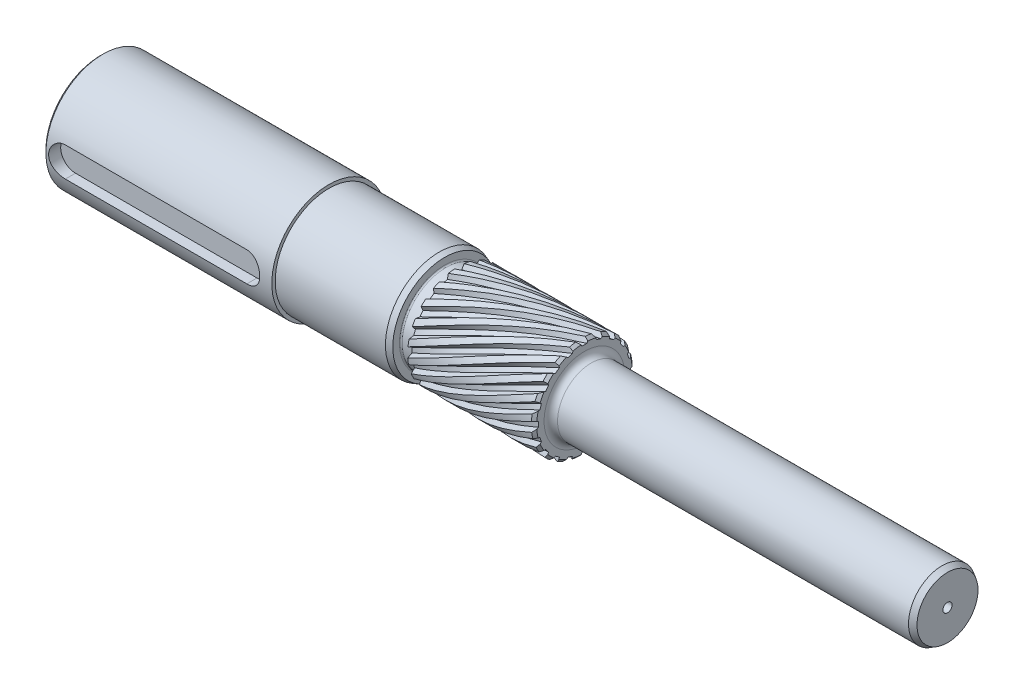
from build123d import *

# Parameters (mm, degrees)
SKETCH_1_R               = 42.5
EXTRUDE_1_DEPTH          = 360
SKETCH_17_OUTSIDE_W      = 162.908
SKETCH_17_OUTSIDE_H      = 162.908
SKETCH_17_OUTSIDE_R      = 40
CUT_EXTRUDE_6_DEPTH      = 190
SKETCH_4_OUTSIDE_W       = 162.908
SKETCH_4_OUTSIDE_H       = 162.908
SKETCH_4_OUTSIDE_R       = 32.5
CUT_EXTRUDE_2_DEPTH      = 10
SKETCH_19_OUTSIDE_W      = 162.908
SKETCH_19_OUTSIDE_H      = 162.908
SKETCH_19_OUTSIDE_R      = 37.5
CUT_EXTRUDE_7_DEPTH      = 94
SKETCH_14_OUTSIDE_W      = 162.908
SKETCH_14_OUTSIDE_H      = 162.908
SKETCH_14_OUTSIDE_R      = 42.5
CUT_EXTRUDE_4_DEPTH      = 360
CUT_EXTRUDE_5_DEPTH      = 9
CHAMFER_1_SIZE           = 2
FILLET_1_R               = 1
CHAMFER_2_SIZE           = 4
CHAMFER_2_SIZE2          = 1.455880937
EXTRUDE_START            = -360
SKETCH_20_R              = 25
EXTRUDE_2_DEPTH          = 270
CHAMFER_3_SIZE           = 4
CHAMFER_3_SIZE2          = 2.309401077
FILLET_2_R               = 5
HOLE_WIZARD_M8_1_D       = 6.8
HOLE_WIZARD_M8_1_DEPTH   = 19.75
HOLE_WIZARD_M8_1_TIP     = 2.042926105
CHAMFER_4_SIZE           = 2
SWEEP_1_PITCH            = 480
SWEEP_1_HEIGHT           = 94
SWEEP_1_RADIUS           = 36
SWEEP_1_START_ANGLE      = -90
PATTERN_CIRCULAR_2_COUNT = 20


with BuildPart() as part:
    # 草图1 → 凸台-拉伸1 (new body)
    with BuildSketch(Plane(origin=(0, 0, 0), x_dir=(0, 0, -1), z_dir=(1, 0, 0))):
        with Locations(Location((0, 0, 0), (0, 0, 180))):
            Circle(SKETCH_1_R)
    extrude(amount=EXTRUDE_1_DEPTH)

    # 草图17 outside → 切除-拉伸6 (cut)
    with BuildSketch(Plane(origin=(360, 0, 0), x_dir=(0, 0, -1), z_dir=(1, 0, 0))):
        Rectangle(SKETCH_17_OUTSIDE_W, SKETCH_17_OUTSIDE_H)
        Circle(SKETCH_17_OUTSIDE_R, mode=Mode.SUBTRACT)
    extrude(amount=-CUT_EXTRUDE_6_DEPTH, mode=Mode.SUBTRACT)

    # 草图4 outside → 切除-拉伸2 (cut)
    with BuildSketch(Plane(origin=(266, 0, 0), x_dir=(0, 0, -1), z_dir=(1, 0, 0))):
        Rectangle(SKETCH_4_OUTSIDE_W, SKETCH_4_OUTSIDE_H)
        Circle(SKETCH_4_OUTSIDE_R, mode=Mode.SUBTRACT)
    extrude(amount=-CUT_EXTRUDE_2_DEPTH, mode=Mode.SUBTRACT)

    # 草图19 outside → 切除-拉伸7 (cut)
    with BuildSketch(Plane(origin=(360, 0, 0), x_dir=(0, 0, -1), z_dir=(1, 0, 0))):
        Rectangle(SKETCH_19_OUTSIDE_W, SKETCH_19_OUTSIDE_H)
        Circle(SKETCH_19_OUTSIDE_R, mode=Mode.SUBTRACT)
    extrude(amount=-CUT_EXTRUDE_7_DEPTH, mode=Mode.SUBTRACT)

    # 草图14 outside → 切除-拉伸4 (cut)
    with BuildSketch(Plane(origin=(360, 0, 0), x_dir=(0, 0, -1), z_dir=(1, 0, 0))):
        Rectangle(SKETCH_14_OUTSIDE_W, SKETCH_14_OUTSIDE_H)
        with Locations(Location((0, 0, 0), (0, 0, 180))):
            Circle(SKETCH_14_OUTSIDE_R, mode=Mode.SUBTRACT)
    extrude(amount=-CUT_EXTRUDE_4_DEPTH, mode=Mode.SUBTRACT)

    # 草图16 → 切除-拉伸5 (cut)
    with BuildSketch(Plane.XY.offset(42.5)):
        with BuildLine():
            Line((15, 11), (150, 11))
            ThreePointArc((150, 11), (161, 0), (150, -11))
            Line((150, -11), (15, -11))
            ThreePointArc((15, -11), (4, 0), (15, 11))
        make_face()
    cut_extrude_5 = extrude(amount=-CUT_EXTRUDE_5_DEPTH, mode=Mode.SUBTRACT)

    # 倒角1
    chamfer_1_edges = [part.edges().sort_by_distance(p)[0] for p in [
        (0, 0, -42.5),
    ]]
    chamfer(chamfer_1_edges, length=CHAMFER_1_SIZE)

    # 镜向1: 切除-拉伸5 across plane
    add(cut_extrude_5.mirror(Plane.XY), mode=Mode.SUBTRACT)

    # 圆角1
    fillet_1_edges = [part.edges().sort_by_distance(p)[0] for p in [
        (256, 0, 32.5),
        (266, 0, 32.5),
    ]]
    fillet(fillet_1_edges, radius=FILLET_1_R)

    # 倒角2
    chamfer_2_edges = [part.edges().sort_by_distance(p)[0] for p in [
        (256, 0, 40),
    ]]
    chamfer_2_side = [part.faces().sort_by_distance(p)[0] for p in [
        (213, 0, 40),
    ]]
    chamfer(chamfer_2_edges, length=CHAMFER_2_SIZE, length2=CHAMFER_2_SIZE2, reference=chamfer_2_side[0])

    # 草图20 → 凸台-拉伸2 (add)
    with BuildSketch(Plane.ZY.offset(EXTRUDE_START)):
        with Locations(Location((0, 0, 0), (0, 0, 180))):
            Circle(SKETCH_20_R)
    extrude(amount=-EXTRUDE_2_DEPTH)

    # 倒角3
    chamfer_3_edges = [part.edges().sort_by_distance(p)[0] for p in [
        (630, 0, 25),
    ]]
    chamfer_3_side = [part.faces().sort_by_distance(p)[0] for p in [
        (495, 0, 25),
    ]]
    chamfer(chamfer_3_edges, length=CHAMFER_3_SIZE, length2=CHAMFER_3_SIZE2, reference=chamfer_3_side[0])

    # 圆角2
    fillet_2_edges = [part.edges().sort_by_distance(p)[0] for p in [
        (360, 0, 25),
    ]]
    fillet(fillet_2_edges, radius=FILLET_2_R)

    # M8 螺纹孔1
    with Locations(Plane(origin=(630, 0, 0), x_dir=(0, 0, -1), z_dir=(1, 0, 0))):
        with Locations((0, 0)):
            Hole(HOLE_WIZARD_M8_1_D / 2, depth=HOLE_WIZARD_M8_1_DEPTH)
            with Locations((0, 0, -(HOLE_WIZARD_M8_1_DEPTH + HOLE_WIZARD_M8_1_TIP / 2))):  # 118° drill point
                Cone(0, HOLE_WIZARD_M8_1_D / 2, HOLE_WIZARD_M8_1_TIP, mode=Mode.SUBTRACT)

    # 倒角4
    chamfer_4_edges = [part.edges().sort_by_distance(p)[0] for p in [
        (360, 0, 37.5),
    ]]
    chamfer(chamfer_4_edges, length=CHAMFER_4_SIZE)

    # 切除-扫描1: sweep along a helix
    with BuildLine() as sweep_1_path:
        add(Helix(SWEEP_1_PITCH, SWEEP_1_HEIGHT, SWEEP_1_RADIUS, center=(360, 0, 0), direction=(-1, 0, 0), lefthand=True, mode=Mode.PRIVATE).rotate(Axis((360, 0, 0), (-1, 0, 0)), SWEEP_1_START_ANGLE))
    # 草图26 → 切除-扫描1 (sweep, cut)
    with BuildSketch(Plane(origin=(360, 0, 0), x_dir=(0, 0, -1), z_dir=(1, 0, 0))):
        Polygon((-1.789637029, 34.25), (1.789637029, 34.25), (3.810362971, 37.75), (-3.810362971, 37.75), align=None)
    sweep_1 = sweep(path=sweep_1_path.line, is_frenet=True, mode=Mode.SUBTRACT)

    # 阵列(圆周)2: 切除-扫描1 ×20 about axis
    pattern_circular_2_axis = Axis((-121.41023433, 0, 0), (1, 0, 0))
    for i in range(1, PATTERN_CIRCULAR_2_COUNT):
        add(sweep_1.rotate(pattern_circular_2_axis, i * 360 / PATTERN_CIRCULAR_2_COUNT), mode=Mode.SUBTRACT)


solid = part.part
